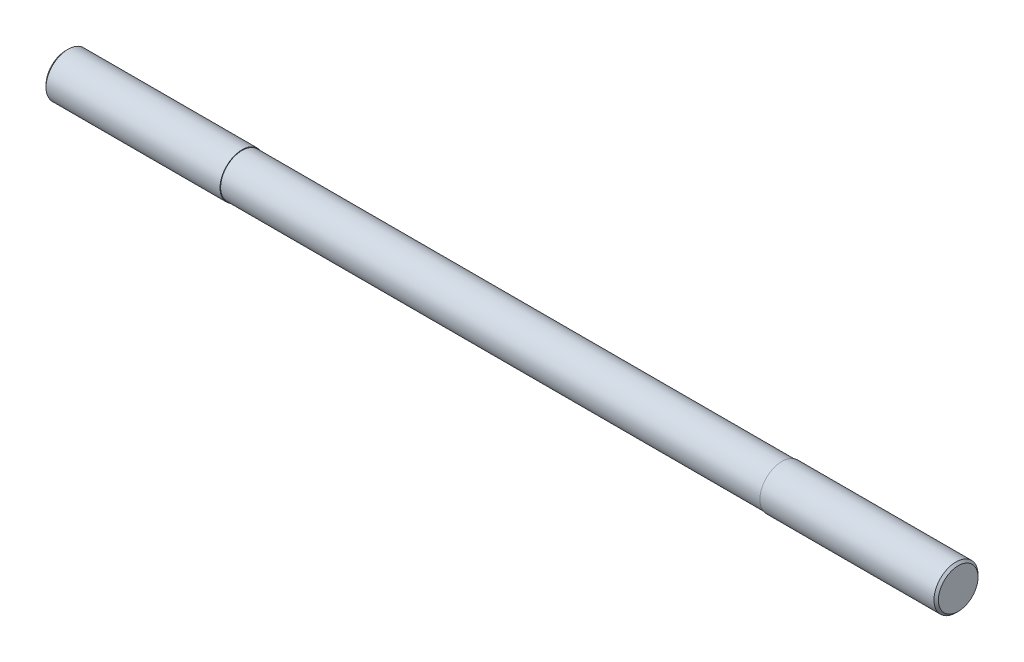
SolidWorks part; units mm, degrees
ref_plane "Front Plane" through (0, 0, 0) normal (0, 0, 1) x (1, 0, 0)
ref_plane "Top Plane" through (0, 0, 0) normal (0, 1, 0) x (1, 0, 0)
ref_plane "Right Plane" through (0, 0, 0) normal (1, 0, 0) x (0, 0, -1)
sketch "Sketch3" plane through (0, 0, 0) normal (0, 0, 1) x (1, 0, 0)
  line L0 (0, 0) -> (132.5429, 0) construction
  line L1 (325, 10) -> (405, 10)
  line L2 (0, 0) -> (405, 0)
  line L3 (0, 0) -> (0, 10)
  line L4 (0, 10) -> (80, 10)
  line L5 (405, 0) -> (405, 10)
  line L7 (80, 10) -> (80, 9.75)
  line L8 (80, 9.75) -> (325, 9.75)
  line L9 (325, 10) -> (325, 9.75)
  dimension "D1" = 20
  dimension "D2" = 19.5
  dimension "D3" = 80
  dimension "D4" = 405
  dimension "D5" = 80
revolve "Revolve1" add sketch "Sketch3" angle 360 about L0
chamfer "Chamfer1" distance 1 angle 45 2 edges at (405, 0, 10) (0, 0, 10)
